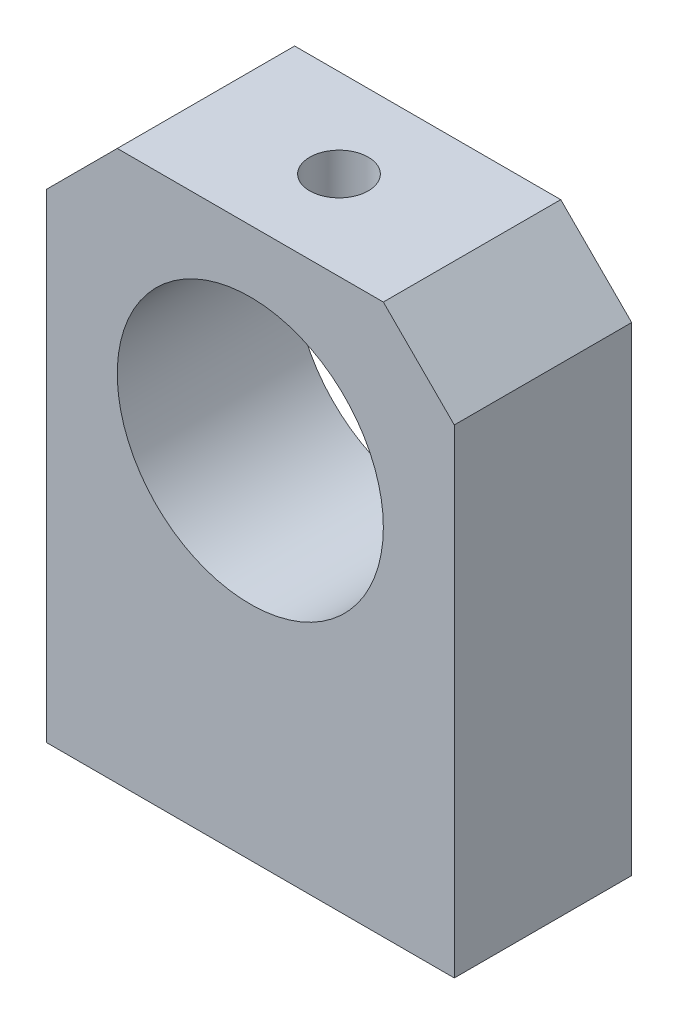
from build123d import *

# Parameters (mm, degrees)
SKETCH_1_W              = 23
SKETCH_1_H              = 31
SKETCH_1_R              = 7.5
EXTRUDE_1_DEPTH         = 5
CHAMFER_1_SIZE          = 4
HOLE_WIZARD_M4_1_REACH  = 35.44
HOLE_WIZARD_M4_1_BORE_R = 1.65
HOLE_WIZARD_M5_2_D      = 4.2
HOLE_WIZARD_M5_2_DEPTH  = 8.4
HOLE_WIZARD_M5_2_TIP    = 1.2618073


with BuildPart() as part:
    # 草图1 → 凸台-拉伸1 (new, symmetric)
    with BuildSketch(Plane.XY):
        with Locations((0, 15.5)):
            Rectangle(SKETCH_1_W, SKETCH_1_H)
        with Locations((0, 20)):
            Circle(SKETCH_1_R, mode=Mode.SUBTRACT)
    extrude(amount=EXTRUDE_1_DEPTH, both=True)

    # 倒角1
    chamfer_1_edges = [part.edges().sort_by_distance(p)[0] for p in [
        (11.5, 31, 0),
        (-11.5, 31, 0),
    ]]
    chamfer(chamfer_1_edges, length=CHAMFER_1_SIZE)

    # M4 螺纹孔1 bore (on position points) → M4 螺纹孔1 (cut, up to next)
    with BuildSketch(Plane.ZX.offset(31), mode=Mode.PRIVATE) as hole_wizard_m4_1_sk1:
        Circle(HOLE_WIZARD_M4_1_BORE_R)
    hole_wizard_m4_1_tool1 = extrude(hole_wizard_m4_1_sk1.sketch, amount=-HOLE_WIZARD_M4_1_REACH, mode=Mode.PRIVATE) & part.part
    add(hole_wizard_m4_1_tool1.solids().sort_by_distance((0, 31, 0))[0], mode=Mode.SUBTRACT)

    # M5 螺纹孔2
    with Locations(Plane(origin=(-6.5, 0, 0), x_dir=(0, 0, -1), z_dir=(0, -1, 0))):
        with Locations((0, 0), (0, 13)):
            Hole(HOLE_WIZARD_M5_2_D / 2, depth=HOLE_WIZARD_M5_2_DEPTH)
            with Locations((0, 0, -(HOLE_WIZARD_M5_2_DEPTH + HOLE_WIZARD_M5_2_TIP / 2))):  # 118° drill point
                Cone(0, HOLE_WIZARD_M5_2_D / 2, HOLE_WIZARD_M5_2_TIP, mode=Mode.SUBTRACT)


solid = part.part
